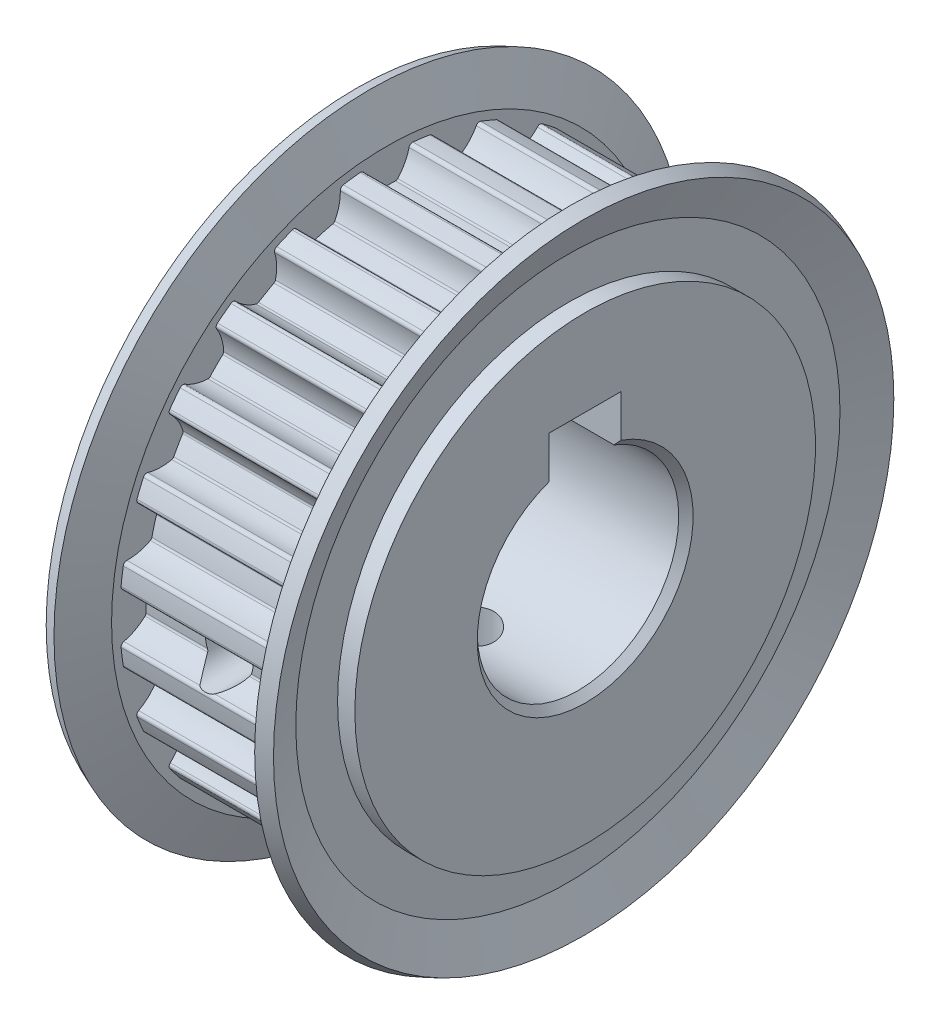
from build123d import *

# Parameters (mm, degrees)
SKETCH2_W          = 12
SKETCH2_H          = 13.5
SKETCH3_W          = 76.4
SKETCH3_H          = 76.4
CUT_EXTRUDE1_DEPTH = 11.6
SKETCH4_R          = 7
CUT_EXTRUDE2_DEPTH = 35.896875427
SKETCH7_W          = 25.120216676
SKETCH7_H          = 8.000541924
CUT_EXTRUDE3_DEPTH = 2.5
SKETCH9_W          = 1.65
SKETCH9_H          = 21.929340102
SKETCH11_W         = 1.65
SKETCH11_H         = 21.929340102
CHAMFER1_SIZE      = 0.5


with BuildPart() as part:
    # Sketch1 → Revolve1 (revolve)
    with BuildSketch(Plane.XY, mode=Mode.PRIVATE) as revolve1_sk:
        Polygon((0, 16), (0, 4.2), (0.2, 4), (27.8, 4), (28, 4.2), (28, 12.3), (27.8, 12.5), (16, 12.5), (16, 16), (14.8, 16), (14.8, 18.901274196), (15.894778254, 21.546988309), (14.970761421, 21.929340102), (13.8, 19.1), (2.2, 19.1), (1.029238579, 21.929340102), (0.105221746, 21.546988309), (1.2, 18.901274196), (1.2, 16), align=None)
    revolve(revolve1_sk.sketch.rotate(Axis((28, 0, 0), (-1, 0, 0)), 270), axis=Axis((28, 0, 0), (-1, 0, 0)))

    # Sketch2 → Cut-Revolve1 (revolve, cut)
    with BuildSketch(Plane.XY, mode=Mode.PRIVATE) as cut_revolve1_sk:
        with Locations((22, 6.75)):
            Rectangle(SKETCH2_W, SKETCH2_H)
    revolve(cut_revolve1_sk.sketch.rotate(Axis((28, 0, 0), (-1, 0, 0)), 270), axis=Axis((28, 0, 0), (-1, 0, 0)), mode=Mode.SUBTRACT)

    # Sketch3 → Cut-Extrude1 (cut)
    with BuildSketch(Plane(origin=(2.2, 0, 0), x_dir=(0, 0, -1), z_dir=(1, 0, 0))):
        Rectangle(SKETCH3_W, SKETCH3_H)
        with BuildLine():
            ThreePointArc((-18.248790316, -1.567329768), (-18.393984043, -1.66562514), (-18.438906438, -1.835110175))
            ThreePointArc((-18.438906438, -1.835110175), (-18.407502372, -2.127147489), (-18.371473281, -2.418650342))
            ThreePointArc((-18.371473281, -2.418650342), (-18.330828224, -2.709545465), (-18.285577409, -2.999759795))
            ThreePointArc((-18.285577409, -2.999759795), (-18.198319753, -3.151843039), (-18.03263263, -3.209210182))
            ThreePointArc((-18.03263263, -3.209210182), (-17.192767769, -3.29562141), (-16.401857339, -3.591088121))
            ThreePointArc((-16.401857339, -3.591088121), (-16.336514808, -3.646161172), (-16.300125243, -3.723481848))
            ThreePointArc((-16.300125243, -3.723481848), (-16.150279816, -4.327454434), (-15.978063469, -4.92543275))
            ThreePointArc((-15.978063469, -4.92543275), (-15.970917412, -5.010589148), (-15.999969127, -5.090955037))
            ThreePointArc((-15.999969127, -5.090955037), (-16.537184324, -5.742291994), (-17.221323071, -6.237058785))
            ThreePointArc((-17.221323071, -6.237058785), (-17.336128728, -6.369583725), (-17.335654474, -6.544920469))
            ThreePointArc((-17.335654474, -6.544920469), (-17.229735656, -6.818878883), (-17.119487737, -7.091124002))
            ThreePointArc((-17.119487737, -7.091124002), (-17.004938429, -7.361587399), (-16.886116502, -7.630201143))
            ThreePointArc((-16.886116502, -7.630201143), (-16.762470039, -7.754518333), (-16.587580861, -7.767047756))
            ThreePointArc((-16.587580861, -7.767047756), (-15.753968828, -7.63314157), (-14.913535605, -7.713837815))
            ThreePointArc((-14.913535605, -7.713837815), (-14.836165611, -7.750122406), (-14.781003927, -7.815390131))
            ThreePointArc((-14.781003927, -7.815390131), (-14.479944751, -8.36), (-14.158828358, -8.893029829))
            ThreePointArc((-14.158828358, -8.893029829), (-14.129885698, -8.973435063), (-14.137147282, -9.058581693))
            ThreePointArc((-14.137147282, -9.058581693), (-14.487478906, -9.8267664), (-15.020251118, -10.481742553))
            ThreePointArc((-15.020251118, -10.481742553), (-15.096844889, -10.639465706), (-15.051006306, -10.808705249))
            ThreePointArc((-15.051006306, -10.808705249), (-14.877790929, -11.045914949), (-14.700837396, -11.28034928))
            ThreePointArc((-14.700837396, -11.28034928), (-14.520190182, -11.511949318), (-14.335894661, -11.740656892))
            ThreePointArc((-14.335894661, -11.740656892), (-14.184285692, -11.828736017), (-14.012112864, -11.795573859))
            ThreePointArc((-14.012112864, -11.795573859), (-13.241562944, -11.450475747), (-12.408881064, -11.310902209))
            ThreePointArc((-12.408881064, -11.310902209), (-12.324756247, -11.325925605), (-12.254581621, -11.374692492))
            ThreePointArc((-12.254581621, -11.374692492), (-11.822825381, -11.822825381), (-11.374692492, -12.254581621))
            ThreePointArc((-11.374692492, -12.254581621), (-11.325925621, -12.324756208), (-11.310902206, -12.40888098))
            ThreePointArc((-11.310902206, -12.40888098), (-11.450475739, -13.241562917), (-11.795573874, -14.012112888))
            ThreePointArc((-11.795573874, -14.012112888), (-11.828736019, -14.184285681), (-11.740656931, -14.335894629))
            ThreePointArc((-11.740656931, -14.335894629), (-11.511949337, -14.520190166), (-11.28034928, -14.700837396))
            ThreePointArc((-11.28034928, -14.700837396), (-11.045914969, -14.877790914), (-10.80870529, -15.051006277))
            ThreePointArc((-10.80870529, -15.051006277), (-10.639465717, -15.09684489), (-10.481742533, -15.020251098))
            ThreePointArc((-10.481742533, -15.020251098), (-9.826766419, -14.487478917), (-9.058581763, -14.137147303))
            ThreePointArc((-9.058581763, -14.137147303), (-8.973435099, -14.129885693), (-8.893029829, -14.158828358))
            ThreePointArc((-8.893029829, -14.158828358), (-8.36, -14.479944751), (-7.815390131, -14.781003927))
            ThreePointArc((-7.815390131, -14.781003927), (-7.750122431, -14.836165578), (-7.713837834, -14.913535522))
            ThreePointArc((-7.713837834, -14.913535522), (-7.633141569, -15.753968799), (-7.767047763, -16.587580886))
            ThreePointArc((-7.767047763, -16.587580886), (-7.754518341, -16.762470022), (-7.630201202, -16.886116475))
            ThreePointArc((-7.630201202, -16.886116475), (-7.361587429, -17.004938416), (-7.091124002, -17.119487737))
            ThreePointArc((-7.091124002, -17.119487737), (-6.818878906, -17.229735647), (-6.544920516, -17.335654457))
            ThreePointArc((-6.544920516, -17.335654457), (-6.369583729, -17.336128729), (-6.237058765, -17.221323034))
            ThreePointArc((-6.237058765, -17.221323034), (-5.742292009, -16.53718434), (-5.090955109, -15.999969172))
            ThreePointArc((-5.090955109, -15.999969172), (-5.01058919, -15.970917417), (-4.92543275, -15.978063469))
            ThreePointArc((-4.92543275, -15.978063469), (-4.327454434, -16.150279816), (-3.723481848, -16.300125243))
            ThreePointArc((-3.723481848, -16.300125243), (-3.646161206, -16.336514782), (-3.59108816, -16.401857264))
            ThreePointArc((-3.59108816, -16.401857264), (-3.295621416, -17.192767742), (-3.209210183, -18.032632658))
            ThreePointArc((-3.209210183, -18.032632658), (-3.151843051, -18.198319739), (-2.999759859, -18.285577398))
            ThreePointArc((-2.999759859, -18.285577398), (-2.709545497, -18.330828219), (-2.418650342, -18.371473281))
            ThreePointArc((-2.418650342, -18.371473281), (-2.127147347, -18.407502388), (-1.83510989, -18.438906467))
            ThreePointArc((-1.83510989, -18.438906467), (-1.665625005, -18.393983948), (-1.567329758, -18.248790274))
            ThreePointArc((-1.567329758, -18.248790274), (-1.266489894, -17.459907982), (-0.776388277, -16.772419583))
            ThreePointArc((-0.776388277, -16.772419583), (-0.706279908, -16.723557512), (-0.622175569, -16.70841996))
            ThreePointArc((-0.622175569, -16.70841996), (0, -16.72), (0.622175569, -16.70841996))
            ThreePointArc((0.622175569, -16.70841996), (0.706279881, -16.723557501), (0.776388237, -16.772419539))
            ThreePointArc((0.776388237, -16.772419539), (1.26648989, -17.459907975), (1.567329768, -18.248790316))
            ThreePointArc((1.567329768, -18.248790316), (1.665625129, -18.393984036), (1.83511015, -18.438906441))
            ThreePointArc((1.83511015, -18.438906441), (2.127147477, -18.407502373), (2.418650342, -18.371473281))
            ThreePointArc((2.418650342, -18.371473281), (2.709545465, -18.330828224), (2.999759795, -18.285577409))
            ThreePointArc((2.999759795, -18.285577409), (3.151843044, -18.198319747), (3.209210182, -18.032632616))
            ThreePointArc((3.209210182, -18.032632616), (3.295621414, -17.19276775), (3.591088132, -16.401857317))
            ThreePointArc((3.591088132, -16.401857317), (3.646161182, -16.3365148), (3.723481848, -16.300125243))
            ThreePointArc((3.723481848, -16.300125243), (4.327454434, -16.150279816), (4.92543275, -15.978063469))
            ThreePointArc((4.92543275, -15.978063469), (5.010589161, -15.970917413), (5.090955058, -15.99996914))
            ThreePointArc((5.090955058, -15.99996914), (5.742292003, -16.537184334), (6.237058785, -17.221323071))
            ThreePointArc((6.237058785, -17.221323071), (6.369583719, -17.336128725), (6.544920456, -17.335654479))
            ThreePointArc((6.544920456, -17.335654479), (6.818878876, -17.229735659), (7.091124002, -17.119487737))
            ThreePointArc((7.091124002, -17.119487737), (7.361587399, -17.004938429), (7.630201143, -16.886116502))
            ThreePointArc((7.630201143, -16.886116502), (7.754518337, -16.762470031), (7.76704775, -16.587580842))
            ThreePointArc((7.76704775, -16.587580842), (7.633141569, -15.753968806), (7.71383782, -14.91353558))
            ThreePointArc((7.71383782, -14.91353558), (7.750122413, -14.836165602), (7.815390131, -14.781003927))
            ThreePointArc((7.815390131, -14.781003927), (8.36, -14.479944751), (8.893029829, -14.158828358))
            ThreePointArc((8.893029829, -14.158828358), (8.97343507, -14.129885697), (9.058581706, -14.137147286))
            ThreePointArc((9.058581706, -14.137147286), (9.826766406, -14.487478909), (10.481742553, -15.020251118))
            ThreePointArc((10.481742553, -15.020251118), (10.639465699, -15.096844888), (10.808705238, -15.051006314))
            ThreePointArc((10.808705238, -15.051006314), (11.045914944, -14.877790933), (11.28034928, -14.700837396))
            ThreePointArc((11.28034928, -14.700837396), (11.511949318, -14.520190182), (11.740656892, -14.335894661))
            ThreePointArc((11.740656892, -14.335894661), (11.828736018, -14.184285685), (11.795573851, -14.012112851))
            ThreePointArc((11.795573851, -14.012112851), (11.450475732, -13.241562897), (11.310902206, -12.40888098))
            ThreePointArc((11.310902206, -12.40888098), (11.325925621, -12.324756208), (11.374692492, -12.254581621))
            ThreePointArc((11.374692492, -12.254581621), (11.822825381, -11.822825381), (12.254581621, -11.374692492))
            ThreePointArc((12.254581621, -11.374692492), (12.324756208, -11.325925621), (12.40888098, -11.310902206))
            ThreePointArc((12.40888098, -11.310902206), (13.241562917, -11.450475739), (14.012112888, -11.795573874))
            ThreePointArc((14.012112888, -11.795573874), (14.184285669, -11.828736021), (14.335894613, -11.740656951))
            ThreePointArc((14.335894613, -11.740656951), (14.520190158, -11.511949347), (14.700837396, -11.28034928))
            ThreePointArc((14.700837396, -11.28034928), (14.877790914, -11.045914969), (15.051006277, -10.80870529))
            ThreePointArc((15.051006277, -10.80870529), (15.096844889, -10.63946571), (15.020251087, -10.481742523))
            ThreePointArc((15.020251087, -10.481742523), (14.487478898, -9.826766388), (14.137147286, -9.058581706))
            ThreePointArc((14.137147286, -9.058581706), (14.129885697, -8.97343507), (14.158828358, -8.893029829))
            ThreePointArc((14.158828358, -8.893029829), (14.479944751, -8.36), (14.781003927, -7.815390131))
            ThreePointArc((14.781003927, -7.815390131), (14.836165578, -7.750122431), (14.913535522, -7.713837833))
            ThreePointArc((14.913535522, -7.713837833), (15.753968799, -7.633141569), (16.587580886, -7.767047763))
            ThreePointArc((16.587580886, -7.767047763), (16.762470017, -7.754518343), (16.886116471, -7.630201212))
            ThreePointArc((16.886116471, -7.630201212), (17.004938414, -7.361587434), (17.119487737, -7.091124002))
            ThreePointArc((17.119487737, -7.091124002), (17.229735647, -6.818878906), (17.335654456, -6.544920516))
            ThreePointArc((17.335654456, -6.544920516), (17.33612873, -6.369583732), (17.22132304, -6.237058768))
            ThreePointArc((17.22132304, -6.237058768), (16.537184343, -5.742292011), (15.999969172, -5.090955109))
            ThreePointArc((15.999969172, -5.090955109), (15.970917417, -5.01058919), (15.978063469, -4.92543275))
            ThreePointArc((15.978063469, -4.92543275), (16.150279816, -4.327454434), (16.300125243, -3.723481848))
            ThreePointArc((16.300125243, -3.723481848), (16.336514782, -3.646161206), (16.401857264, -3.59108816))
            ThreePointArc((16.401857264, -3.59108816), (17.192767742, -3.295621416), (18.032632658, -3.209210183))
            ThreePointArc((18.032632658, -3.209210183), (18.198319734, -3.151843054), (18.285577396, -2.99975987))
            ThreePointArc((18.285577396, -2.99975987), (18.330828218, -2.709545503), (18.371473281, -2.418650342))
            ThreePointArc((18.371473281, -2.418650342), (18.407502388, -2.127147347), (18.438906467, -1.83510989))
            ThreePointArc((18.438906467, -1.83510989), (18.393983949, -1.665625007), (18.248790278, -1.567329758))
            ThreePointArc((18.248790278, -1.567329758), (17.459907958, -1.266489881), (16.772419539, -0.776388237))
            ThreePointArc((16.772419539, -0.776388237), (16.723557501, -0.706279881), (16.70841996, -0.622175569))
            ThreePointArc((16.70841996, -0.622175569), (16.72, 0), (16.70841996, 0.622175569))
            ThreePointArc((16.70841996, 0.622175569), (16.723557501, 0.706279881), (16.772419539, 0.776388237))
            ThreePointArc((16.772419539, 0.776388237), (17.459907975, 1.26648989), (18.248790316, 1.567329768))
            ThreePointArc((18.248790316, 1.567329768), (18.393984036, 1.665625129), (18.438906441, 1.83511015))
            ThreePointArc((18.438906441, 1.83511015), (18.407502373, 2.127147477), (18.371473281, 2.418650342))
            ThreePointArc((18.371473281, 2.418650342), (18.330828199, 2.709545632), (18.285577354, 2.999760128))
            ThreePointArc((18.285577354, 2.999760128), (18.198319619, 3.15184315), (18.03263262, 3.209210182))
            ThreePointArc((18.03263262, 3.209210182), (17.192767752, 3.295621414), (16.401857317, 3.591088132))
            ThreePointArc((16.401857317, 3.591088132), (16.3365148, 3.646161182), (16.300125243, 3.723481848))
            ThreePointArc((16.300125243, 3.723481848), (16.150279816, 4.327454434), (15.978063469, 4.92543275))
            ThreePointArc((15.978063469, 4.92543275), (15.970917413, 5.010589161), (15.99996914, 5.090955058))
            ThreePointArc((15.99996914, 5.090955058), (16.537184334, 5.742292003), (17.221323071, 6.237058785))
            ThreePointArc((17.221323071, 6.237058785), (17.336128723, 6.369583713), (17.335654483, 6.544920446))
            ThreePointArc((17.335654483, 6.544920446), (17.229735661, 6.818878871), (17.119487737, 7.091124002))
            ThreePointArc((17.119487737, 7.091124002), (17.004938362, 7.361587554), (16.886116363, 7.63020145))
            ThreePointArc((16.886116363, 7.63020145), (16.762469882, 7.754518405), (16.587580851, 7.767047753))
            ThreePointArc((16.587580851, 7.767047753), (15.753968751, 7.633141568), (14.913535464, 7.713837847))
            ThreePointArc((14.913535464, 7.713837847), (14.836165554, 7.75012245), (14.781003927, 7.815390131))
            ThreePointArc((14.781003927, 7.815390131), (14.479944751, 8.36), (14.158828358, 8.893029829))
            ThreePointArc((14.158828358, 8.893029829), (14.129885697, 8.97343507), (14.137147286, 9.058581706))
            ThreePointArc((14.137147286, 9.058581706), (14.487478909, 9.826766406), (15.020251118, 10.481742553))
            ThreePointArc((15.020251118, 10.481742553), (15.096844887, 10.639465688), (15.051006327, 10.808705221))
            ThreePointArc((15.051006327, 10.808705221), (14.87779094, 11.045914935), (14.700837396, 11.28034928))
            ThreePointArc((14.700837396, 11.28034928), (14.520190077, 11.51194945), (14.335894448, 11.740657153))
            ThreePointArc((14.335894448, 11.740657153), (14.184285527, 11.828736045), (14.012112865, 11.79557386))
            ThreePointArc((14.012112865, 11.79557386), (13.241562905, 11.450475735), (12.40888098, 11.310902206))
            ThreePointArc((12.40888098, 11.310902206), (12.324756208, 11.325925621), (12.254581621, 11.374692492))
            ThreePointArc((12.254581621, 11.374692492), (11.822825381, 11.822825381), (11.374692492, 12.254581621))
            ThreePointArc((11.374692492, 12.254581621), (11.325925621, 12.324756208), (11.310902206, 12.40888098))
            ThreePointArc((11.310902206, 12.40888098), (11.450475739, 13.241562917), (11.795573874, 14.012112888))
            ThreePointArc((11.795573874, 14.012112888), (11.828736022, 14.184285664), (11.740656958, 14.335894607))
            ThreePointArc((11.740656958, 14.335894607), (11.511949351, 14.520190155), (11.28034928, 14.700837396))
            ThreePointArc((11.28034928, 14.700837396), (11.045914834, 14.877791015), (10.808705017, 15.051006474))
            ThreePointArc((10.808705017, 15.051006474), (10.639465544, 15.096844873), (10.481742526, 15.02025109))
            ThreePointArc((10.481742526, 15.02025109), (9.826766389, 14.487478899), (9.058581706, 14.137147286))
            ThreePointArc((9.058581706, 14.137147286), (8.97343507, 14.129885697), (8.893029829, 14.158828358))
            ThreePointArc((8.893029829, 14.158828358), (8.36, 14.479944751), (7.815390131, 14.781003927))
            ThreePointArc((7.815390131, 14.781003927), (7.750122431, 14.836165578), (7.713837833, 14.913535522))
            ThreePointArc((7.713837833, 14.913535522), (7.633141569, 15.753968799), (7.767047763, 16.587580886))
            ThreePointArc((7.767047763, 16.587580886), (7.754518348, 16.762470007), (7.630201233, 16.886116461))
            ThreePointArc((7.630201233, 16.886116461), (7.361587444, 17.004938409), (7.091124002, 17.119487737))
            ThreePointArc((7.091124002, 17.119487737), (6.818878749, 17.229735709), (6.544920201, 17.335654576))
            ThreePointArc((6.544920201, 17.335654576), (6.369583574, 17.336128672), (6.237058768, 17.22132304))
            ThreePointArc((6.237058768, 17.22132304), (5.74229197, 16.537184299), (5.090955008, 15.999969109))
            ThreePointArc((5.090955008, 15.999969109), (5.010589131, 15.970917409), (4.92543275, 15.978063469))
            ThreePointArc((4.92543275, 15.978063469), (4.327454434, 16.150279816), (3.723481848, 16.300125243))
            ThreePointArc((3.723481848, 16.300125243), (3.646161206, 16.336514782), (3.59108816, 16.401857264))
            ThreePointArc((3.59108816, 16.401857264), (3.295621416, 17.192767742), (3.209210183, 18.032632658))
            ThreePointArc((3.209210183, 18.032632658), (3.151843062, 18.198319726), (2.999759892, 18.285577393))
            ThreePointArc((2.999759892, 18.285577393), (2.709545514, 18.330828217), (2.418650342, 18.371473281))
            ThreePointArc((2.418650342, 18.371473281), (2.127147514, 18.407502369), (1.835110225, 18.438906433))
            ThreePointArc((1.835110225, 18.438906433), (1.66562516, 18.393984058), (1.567329768, 18.248790316))
            ThreePointArc((1.567329768, 18.248790316), (1.266489876, 17.459907949), (0.776388196, 16.772419496))
            ThreePointArc((0.776388196, 16.772419496), (0.706279853, 16.72355749), (0.622175569, 16.70841996))
            ThreePointArc((0.622175569, 16.70841996), (0, 16.72), (-0.622175569, 16.70841996))
            ThreePointArc((-0.622175569, 16.70841996), (-0.706279881, 16.723557501), (-0.776388237, 16.772419539))
            ThreePointArc((-0.776388237, 16.772419539), (-1.26648989, 17.459907975), (-1.567329768, 18.248790316))
            ThreePointArc((-1.567329768, 18.248790316), (-1.665625155, 18.393984054), (-1.835110211, 18.438906435))
            ThreePointArc((-1.835110211, 18.438906435), (-2.127147507, 18.40750237), (-2.418650342, 18.371473281))
            ThreePointArc((-2.418650342, 18.371473281), (-2.709545465, 18.330828224), (-2.999759795, 18.285577409))
            ThreePointArc((-2.999759795, 18.285577409), (-3.15184303, 18.198319764), (-3.209210183, 18.032632658))
            ThreePointArc((-3.209210183, 18.032632658), (-3.29562141, 17.192767771), (-3.591088132, 16.401857317))
            ThreePointArc((-3.591088132, 16.401857317), (-3.646161182, 16.3365148), (-3.723481848, 16.300125243))
            ThreePointArc((-3.723481848, 16.300125243), (-4.327454434, 16.150279816), (-4.92543275, 15.978063469))
            ThreePointArc((-4.92543275, 15.978063469), (-5.010589161, 15.970917413), (-5.090955058, 15.99996914))
            ThreePointArc((-5.090955058, 15.99996914), (-5.742292003, 16.537184334), (-6.237058785, 17.221323071))
            ThreePointArc((-6.237058785, 17.221323071), (-6.369583742, 17.336128734), (-6.544920503, 17.335654461))
            ThreePointArc((-6.544920503, 17.335654461), (-6.8188789, 17.22973565), (-7.091124002, 17.119487737))
            ThreePointArc((-7.091124002, 17.119487737), (-7.361587399, 17.004938429), (-7.630201143, 16.886116502))
            ThreePointArc((-7.630201143, 16.886116502), (-7.75451833, 16.762470044), (-7.767047759, 16.587580871))
            ThreePointArc((-7.767047759, 16.587580871), (-7.63314157, 15.753968834), (-7.713837815, 14.913535605))
            ThreePointArc((-7.713837815, 14.913535605), (-7.750122406, 14.836165611), (-7.815390131, 14.781003927))
            ThreePointArc((-7.815390131, 14.781003927), (-8.36, 14.479944751), (-8.893029829, 14.158828358))
            ThreePointArc((-8.893029829, 14.158828358), (-8.973435063, 14.129885698), (-9.058581693, 14.137147282))
            ThreePointArc((-9.058581693, 14.137147282), (-9.8267664, 14.487478906), (-10.481742553, 15.020251118))
            ThreePointArc((-10.481742553, 15.020251118), (-10.639465706, 15.096844889), (-10.808705249, 15.051006306))
            ThreePointArc((-10.808705249, 15.051006306), (-11.045914949, 14.877790929), (-11.28034928, 14.700837396))
            ThreePointArc((-11.28034928, 14.700837396), (-11.511949318, 14.520190182), (-11.740656892, 14.335894661))
            ThreePointArc((-11.740656892, 14.335894661), (-11.828736016, 14.184285699), (-11.795573866, 14.012112875))
            ThreePointArc((-11.795573866, 14.012112875), (-11.450475749, 13.241562951), (-11.310902209, 12.408881064))
            ThreePointArc((-11.310902209, 12.408881064), (-11.325925605, 12.324756247), (-11.374692492, 12.254581621))
            ThreePointArc((-11.374692492, 12.254581621), (-11.822825381, 11.822825381), (-12.254581621, 11.374692492))
            ThreePointArc((-12.254581621, 11.374692492), (-12.324756208, 11.325925621), (-12.40888098, 11.310902206))
            ThreePointArc((-12.40888098, 11.310902206), (-13.241562917, 11.450475739), (-14.012112888, 11.795573874))
            ThreePointArc((-14.012112888, 11.795573874), (-14.184285681, 11.828736019), (-14.335894629, 11.740656931))
            ThreePointArc((-14.335894629, 11.740656931), (-14.520190166, 11.511949337), (-14.700837396, 11.28034928))
            ThreePointArc((-14.700837396, 11.28034928), (-14.877790914, 11.045914969), (-15.051006277, 10.80870529))
            ThreePointArc((-15.051006277, 10.80870529), (-15.09684489, 10.639465717), (-15.020251098, 10.481742533))
            ThreePointArc((-15.020251098, 10.481742533), (-14.487478917, 9.826766419), (-14.137147303, 9.058581763))
            ThreePointArc((-14.137147303, 9.058581763), (-14.129885693, 8.973435099), (-14.158828358, 8.893029829))
            ThreePointArc((-14.158828358, 8.893029829), (-14.479944751, 8.36), (-14.781003927, 7.815390131))
            ThreePointArc((-14.781003927, 7.815390131), (-14.836165578, 7.750122431), (-14.913535522, 7.713837833))
            ThreePointArc((-14.913535522, 7.713837833), (-15.753968799, 7.633141569), (-16.587580886, 7.767047763))
            ThreePointArc((-16.587580886, 7.767047763), (-16.762470028, 7.754518338), (-16.886116481, 7.630201189))
            ThreePointArc((-16.886116481, 7.630201189), (-17.004938419, 7.361587423), (-17.119487737, 7.091124002))
            ThreePointArc((-17.119487737, 7.091124002), (-17.229735647, 6.818878906), (-17.335654456, 6.544920516))
            ThreePointArc((-17.335654456, 6.544920516), (-17.336128732, 6.369583736), (-17.221323046, 6.237058771))
            ThreePointArc((-17.221323046, 6.237058771), (-16.537184354, 5.742292022), (-15.999969185, 5.09095513))
            ThreePointArc((-15.999969185, 5.09095513), (-15.970917419, 5.010589202), (-15.978063469, 4.92543275))
            ThreePointArc((-15.978063469, 4.92543275), (-16.150279816, 4.327454434), (-16.300125243, 3.723481848))
            ThreePointArc((-16.300125243, 3.723481848), (-16.33651478, 3.646161208), (-16.401857258, 3.591088164))
            ThreePointArc((-16.401857258, 3.591088164), (-17.192767738, 3.295621417), (-18.032632658, 3.209210183))
            ThreePointArc((-18.032632658, 3.209210183), (-18.198319744, 3.151843046), (-18.285577401, 2.999759845))
            ThreePointArc((-18.285577401, 2.999759845), (-18.33082822, 2.70954549), (-18.371473281, 2.418650342))
            ThreePointArc((-18.371473281, 2.418650342), (-18.407502369, 2.127147514), (-18.438906433, 1.835110225))
            ThreePointArc((-18.438906433, 1.835110225), (-18.393984051, 1.66562515), (-18.24879029, 1.567329761))
            ThreePointArc((-18.24879029, 1.567329761), (-17.459908001, 1.266489904), (-16.772419601, 0.776388294))
            ThreePointArc((-16.772419601, 0.776388294), (-16.723557517, 0.70627992), (-16.70841996, 0.622175569))
            ThreePointArc((-16.70841996, 0.622175569), (-16.72, 0), (-16.70841996, -0.622175569))
            ThreePointArc((-16.70841996, -0.622175569), (-16.7235575, -0.706279877), (-16.772419534, -0.776388232))
            ThreePointArc((-16.772419534, -0.776388232), (-17.459907972, -1.266489888), (-18.248790316, -1.567329768))
        make_face(mode=Mode.SUBTRACT)
    extrude(amount=CUT_EXTRUDE1_DEPTH, mode=Mode.SUBTRACT)

    # Sketch4 → Cut-Extrude2 (cut, through all)
    with BuildSketch(Plane(origin=(16, 0, 0), x_dir=(0, 0, -1), z_dir=(1, 0, 0))):
        Circle(SKETCH4_R)
    extrude(amount=-CUT_EXTRUDE2_DEPTH, mode=Mode.SUBTRACT)

    # Sketch7 → Cut-Extrude3 (cut, symmetric)
    with BuildSketch(Plane.XY):
        with Locations((6.91723204, 5.999729038)):
            Rectangle(SKETCH7_W, SKETCH7_H)
    extrude(amount=CUT_EXTRUDE3_DEPTH, both=True, mode=Mode.SUBTRACT)

    # Sketch9 → M4 Tapped Hole1 (revolve, cut)
    with BuildSketch(Plane(origin=(8, 0, 0), x_dir=(0, 0, 1), z_dir=(1, 0, 0))):
        with Locations((0.825, 10.964670051)):
            Rectangle(SKETCH9_W, SKETCH9_H)
    revolve(axis=Axis((8, 6.35, 0), (0, -1, 0)), mode=Mode.SUBTRACT)

    # Sketch11 → M4 Tapped Hole2 (revolve, cut)
    with BuildSketch(Plane.YZ.offset(8)):
        with Locations((0.825, 10.964670051)):
            Rectangle(SKETCH11_W, SKETCH11_H)
    revolve(axis=Axis((8, 0, -6.35), (0, 0, 1)), mode=Mode.SUBTRACT)

    # Chamfer1
    chamfer1_edges = [part.edges().sort_by_distance(p)[0] for p in [
        (0, -7, 0),
        (16, -7, 0),
    ]]
    chamfer(chamfer1_edges, length=CHAMFER1_SIZE)


solid = part.part
